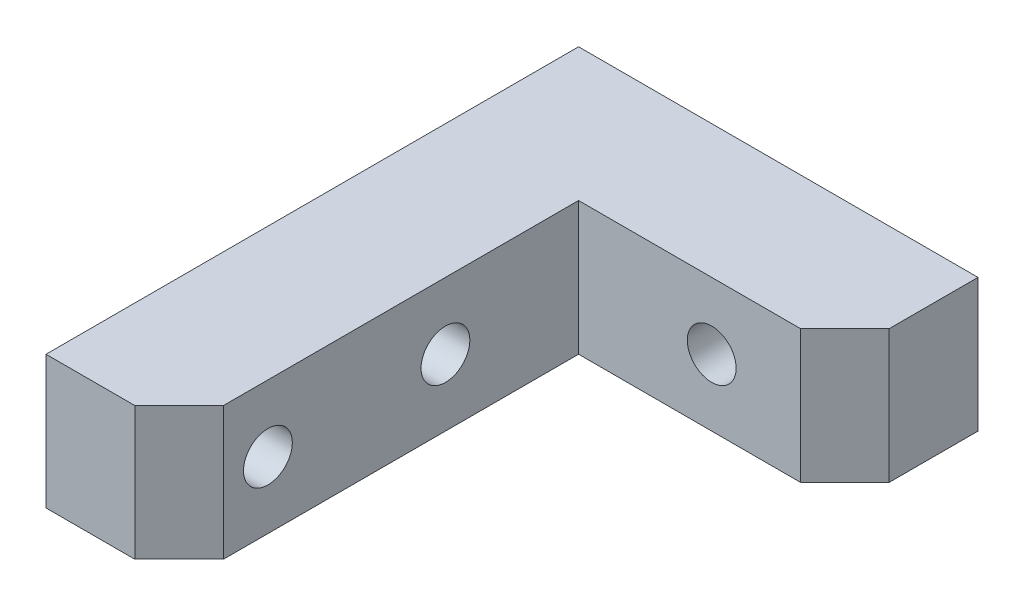
from build123d import *

# Parameters (mm, degrees)
EXTRUDE_1_DEPTH         = 7.5
CHAMFER_1_SIZE          = 5
HOLE_WIZARD_5_5_5_5_1_D = 5.5
HOLE_WIZARD_5_5_5_5_2_D = 5.5


with BuildPart() as part:
    # 草图1 → 凸台-拉伸1 (new, symmetric)
    with BuildSketch(Plane(origin=(0, 0, 0), x_dir=(1, 0, 0), z_dir=(0, 1, 0))):
        Polygon((30, 0), (0, 0), (0, -45), (-15, -45), (-15, 15), (30, 15), align=None)
    extrude(amount=EXTRUDE_1_DEPTH, both=True)

    # 倒角1
    chamfer_1_edges = [part.edges().sort_by_distance(p)[0] for p in [
        (30, 0, 0),
        (0, 0, 45),
    ]]
    chamfer(chamfer_1_edges, length=CHAMFER_1_SIZE)

    # Ø5.5 (5.5) 直径孔1 (through all)
    with Locations(Plane(origin=(0, 0, 0), x_dir=(0, 0, -1), z_dir=(1, 0, 0))):
        with Locations((-35, 0), (-15, 0)):
            Hole(HOLE_WIZARD_5_5_5_5_1_D / 2)

    # Ø5.5 (5.5) 直径孔2 (through all)
    with Locations(Plane.XY):
        with Locations((15, 0)):
            Hole(HOLE_WIZARD_5_5_5_5_2_D / 2)


solid = part.part
